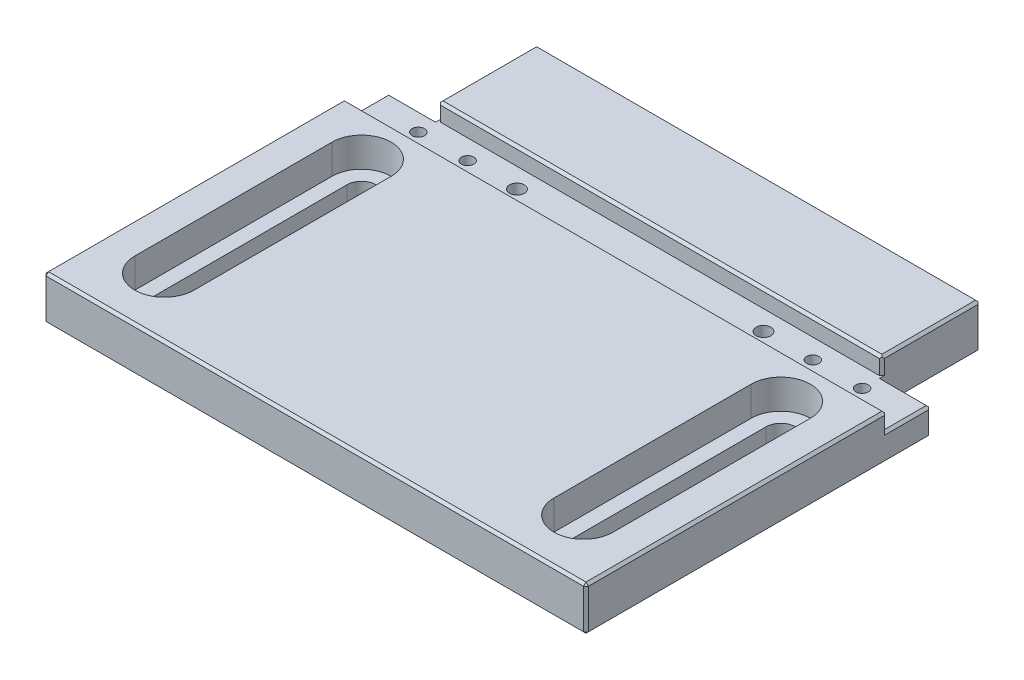
SolidWorks part; units mm, degrees
ref_plane "Front Plane" through (0, 0, 0) normal (0, 0, 1) x (1, 0, 0)
ref_plane "Top Plane" through (0, 0, 0) normal (0, 1, 0) x (1, 0, 0)
ref_plane "Right Plane" through (0, 0, 0) normal (1, 0, 0) x (0, 0, -1)
other "Configuration Table"
sketch "Sketch1" plane through (0, 0, 0) normal (0, 1, 0) x (1, 0, 0)
  line L1 (0, 0) -> (110, 0)
  line L2 (0, 0) -> (0, 90)
  line L3 (0, 90) -> (110, 90)
  line L4 (110, 0) -> (110, 90)
  dimension "D1" = 90
  dimension "D2" = 110
extrude "Boss-Extrude1" add sketch "Sketch1" along normal blind 9
sketch "Sketch2" plane through (0, 9, 0) normal (0, 1, 0) x (1, 0, 0)
  line L0 (0, 90) -> (0, 0) construction
  line L1 (0, 70) -> (110, 70)
  line L2 (0, 70) -> (0, 62)
  line L3 (0, 62) -> (110, 62)
  line L4 (110, 70) -> (110, 62)
  line L5 (110, 0) -> (110, 90) construction
  line L6 (110, 90) -> (0, 90) construction
  dimension "D1" = 20
  dimension "D2" = 8
extrude "Boss-Extrude2" add sketch "Sketch2" along normal blind 1.5
sketch "Sketch5" plane through (0, 0, 0) normal (0, -1, 0) x (1, 0, 0)
  line L1 (0, -90) -> (20, -90)
  line L2 (0, -90) -> (0, -110)
  line L3 (0, -110) -> (20, -110)
  line L4 (20, -90) -> (20, -110)
  line L5 (110, -90) -> (90, -90)
  line L6 (110, -90) -> (110, -110)
  line L7 (110, -110) -> (90, -110)
  line L8 (90, -90) -> (90, -110)
  dimension "D1" = 70
  dimension "D2" = 20
  dimension "D3" = 20
  dimension "D4" = 20
extrude "Boss-Extrude3" add sketch "Sketch5" against normal up to surface (9 mm away) up to face at (55, 9, -80)
sketch "Sketch3" plane through (0, 9, 0) normal (0, 1, 0) x (1, 0, 0)
  line L0 (12.5, 52) -> (12.5, 12) construction
  line L1 (15.5, 52) -> (15.5, 12)
  line L2 (9.5, 52) -> (9.5, 12)
  line L3 (0, 0) -> (110, 0) construction
  line L5 (12.5, 75) -> (97.5, 75) construction
  line L6 (0, 62) -> (110, 62) construction
  line L7 (90, 90) -> (20, 90) construction
  line L8 (94.5, 52) -> (94.5, 12)
  line L9 (100.5, 52) -> (100.5, 12)
  line L10 (97.5, 52) -> (97.5, 12) construction
  arc A0 (15.5, 52) -> (9.5, 52) centre (12.5, 52) ccw
  arc A1 (9.5, 12) -> (15.5, 12) centre (12.5, 12) ccw
  arc A2 (100.5, 52) -> (94.5, 52) centre (97.5, 52) ccw
  arc A3 (94.5, 12) -> (100.5, 12) centre (97.5, 12) ccw
  point P2 (12.5, 32)
  point P13 (55, 62)
  point P14 (55, 75)
  point P21 (97.5, 32)
  dimension "D1" = 6
  dimension "D2" = 40
  dimension "D3" = 52
  dimension "D4" = 85
  dimension "D5" = 15
  dimension "D6" = 2
extrude "Cut-Extrude1" cut sketch "Sketch3" against normal through all
sketch "Sketch4" plane through (0, 9, 0) normal (0, 1, 0) x (1, 0, 0)
  line L7 (6.5, 52) -> (6.5, 12)
  line L8 (18.5, 12) -> (18.5, 52)
  line L9 (6.5, 52) -> (6.5, 12)
  line L10 (18.5, 12) -> (18.5, 52)
  line L12 (103.5, 12) -> (103.5, 52)
  line L13 (91.5, 52) -> (91.5, 12)
  line L14 (103.5, 12) -> (103.5, 52)
  line L15 (91.5, 52) -> (91.5, 12)
  arc A2 (18.5, 52) -> (6.5, 52) centre (12.5, 52) ccw
  arc A3 (18.5, 52) -> (6.5, 52) centre (12.5, 52) ccw
  arc A5 (6.5, 12) -> (18.5, 12) centre (12.5, 12) ccw
  arc A6 (6.5, 12) -> (18.5, 12) centre (12.5, 12) ccw
  arc A12 (91.5, 12) -> (103.5, 12) centre (97.5, 12) ccw
  arc A13 (103.5, 52) -> (91.5, 52) centre (97.5, 52) ccw
  arc A14 (91.5, 12) -> (103.5, 12) centre (97.5, 12) ccw
  arc A15 (103.5, 52) -> (91.5, 52) centre (97.5, 52) ccw
  dimension "D1" = 3
  dimension "D2" = 3
  dimension "D3" = 3
extrude "Cut-Extrude2" cut sketch "Sketch4" against normal blind 6
sketch "Sketch6" plane through (0, 9, 0) normal (0, 1, 0) x (1, 0, 0)
  line L0 (20, 110) -> (0, 110) construction
  line L1 (0, 70) -> (10, 70)
  line L2 (0, 70) -> (0, 110)
  line L3 (0, 110) -> (10, 110)
  line L4 (10, 70) -> (10, 110)
  line L6 (55, 90) -> (55, 70) construction
  line L7 (90, 90) -> (20, 90) construction
  line L8 (110, 70) -> (0, 70) construction
  line L9 (100, 70) -> (100, 110)
  line L10 (110, 110) -> (100, 110)
  line L11 (110, 70) -> (110, 110)
  line L12 (110, 70) -> (100, 70)
  dimension "D1" = 10
extrude "Cut-Extrude3" cut sketch "Sketch6" against normal through all
sketch "Sketch8" plane through (0, 10.5, 0) normal (0, 1, 0) x (1, 0, 0)
  line L0 (110, 0) -> (110, 62) construction
  line L1 (0, 70) -> (110, 70)
  line L2 (0, 70) -> (0, 61)
  line L3 (0, 61) -> (110, 61)
  line L4 (110, 70) -> (110, 61)
  dimension "D1" = 9
extrude "Cut-Extrude5" cut sketch "Sketch8" against normal blind 5
sketch "Sketch10" plane through (0, 5.5, 0) normal (0, 1, 0) x (1, 0, 0)
  line L0 (0, 70) -> (0, 61) construction
  line L1 (110, 61) -> (110, 70) construction
  line L2 (10, 70) -> (0, 70) construction
  point P0 (10, 66)
  point P1 (100, 66)
  point P9 (20, 66)
  point P11 (90, 66)
  dimension "D1" = 90
  dimension "D2" = 10
  dimension "D3" = 10
  dimension "D4" = 4
  dimension "D5" = 10
  dimension "D6" = 10
hole_wizard "M3 Tapped Hole1" positions "Sketch10" profile "Sketch11" tap size "M3" standard "GB" end condition through all
sketch "Sketch11" plane through (10, 5.5, -66) normal (1, 0, 0) x (0, 0, 1)
  line L0 (0, 0) -> (0, 5.5)
  line L1 (0, 5.5) -> (1.25, 5.5)
  line L2 (1.25, 5.5) -> (1.25, 0)
  line L5 (1.25, 0) -> (0, 0)
  line L11 (0, -6.35) -> (0, 107.95) construction
  dimension "通孔螺纹孔钻头直径" = 2.5
  dimension "通孔螺纹孔钻头深度" = 5.5
cosmetic thread "Hole thread1" parameters "D2"=3
cosmetic thread "Hole thread2" parameters "D2"=3
cosmetic thread "Hole thread3" parameters "D2"=3
cosmetic thread "Hole thread4" parameters "D2"=3
other "Move Face1" face at (95, 4.5, -110) face at (15, 4.5, -110) parameters "D1"=20
sketch "Sketch12" plane through (0, 5.5, 0) normal (0, 1, 0) x (1, 0, 0)
  line L0 (100, 70) -> (10, 70) construction
  circle A0 centre (20, 66) radius 1.25 construction
  circle A1 centre (90, 66) radius 1.25 construction
  point P0 (30, 66)
  point P1 (80, 66)
  dimension "D2" = 10
  dimension "D1" = 4
  dimension "D3" = 10
hole_wizard "Ø3.0mm dowel hole1" positions "Sketch12" profile "Sketch13" hole size "Ø3.0" standard "GB" end condition through all
sketch "Sketch13" plane through (30, 5.5, -66) normal (1, 0, 0) x (0, 0, 1)
  line L0 (0, 0) -> (0, 5.5)
  line L1 (0, 5.5) -> (1.5, 5.5)
  line L2 (1.5, 5.5) -> (1.5, 0)
  line L5 (1.5, 0) -> (0, 0)
  line L11 (0, -6.35) -> (0, 107.95) construction
  dimension "通孔孔直径" = 3
  dimension "通孔孔深度" = 5.5
chamfer "Chamfer1" distance 0.5 18 edges at (0, 0, -35) (110, 9, -30.5) (10, 4.5, -90) (100, 4.5, -90) (110, 2.75, -70) (0, 2.75, -70) (0, 9, -30.5) (110, 7.25, -61) (0, 7.25, -61) (0, 5.5, -65.5) (110, 5.5, -65.5) (55, 9, -90) (55, 0, -90) (110, 0, -35) (55, 0, 0) (110, 4.5, 0) (0, 4.5, 0) (55, 9, 0)
chamfer "Chamfer3" distance 0.5 10 edges at (100, 0, -79.75) (100, 9, -79.75) (10, 0, -79.75) (10, 9, -79.75) (104.75, 0, -70) (5.25, 0, -70) (55, 9, -61) (55, 9, -70) (5.25, 5.5, -70) (104.75, 5.5, -70)
chamfer "Chamfer4" distance 0.5 2 edges at (10, 7, -70) (100, 7, -70)
